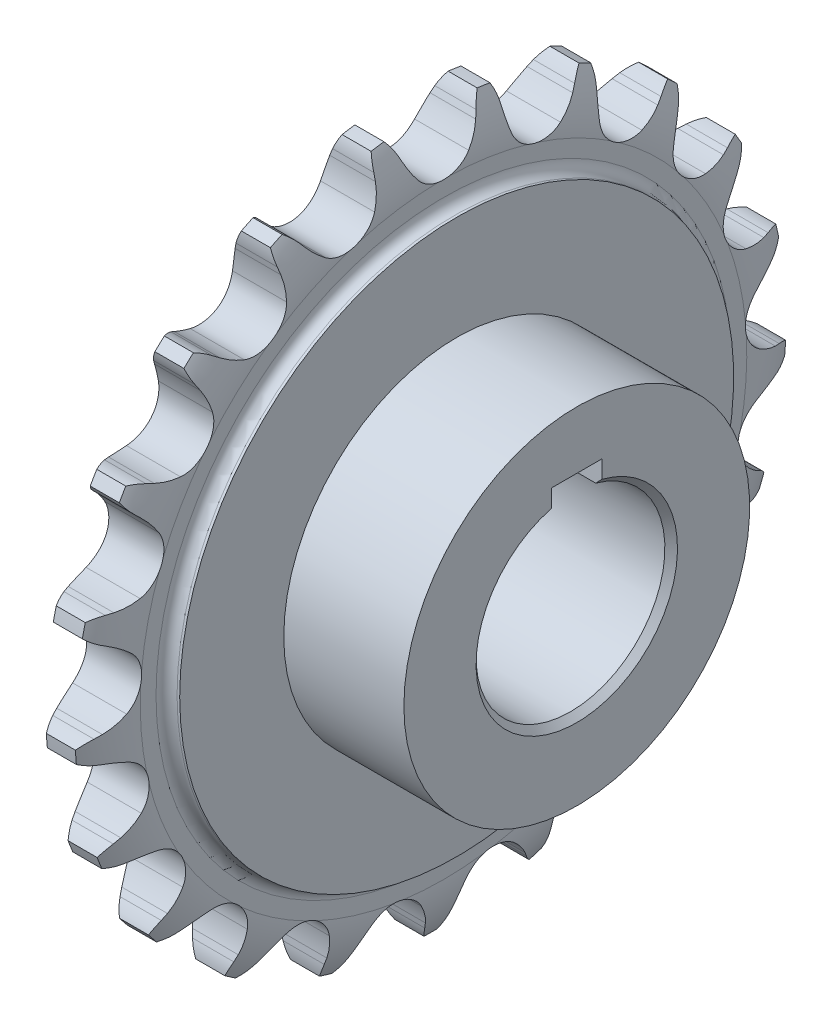
from build123d import *

# Parameters (mm, degrees)
CUT_EXTRUDE_1_DEPTH      = 6.459352492
PATTERN_CIRCULAR_1_COUNT = 21
SKETCH_3_W               = 19.081295016
SKETCH_3_H               = 12.4651341
SKETCH_4_W               = 8
SKETCH_4_H               = 3.843167657
CUT_EXTRUDE_2_DEPTH      = 87.013388292
CHAMFER_1_SIZE           = 1
CHAMFER_3_SIZE           = 1


with BuildPart() as part:
    # 草图1 → 旋转1 (revolve)
    with BuildSketch(Plane.XY, mode=Mode.PRIVATE) as revolve_1_sk:
        with BuildLine():
            Line((-6.459352492, 15), (-6.459352492, 44))
            Line((-6.459352492, 44), (-6.041681994, 44))
            ThreePointArc((-6.041681994, 44), (-4.860331427, 44.489331427), (-4.371, 45.670681994))
            Line((-4.371, 45.670681994), (-4.371, 48.176704985))
            ThreePointArc((-4.371, 48.176704985), (-3.911774122, 52.480340085), (-2.30725, 56.5))
            Line((-2.30725, 56.5), (2.30725, 56.5))
            ThreePointArc((2.30725, 56.5), (3.911774122, 52.480340085), (4.371, 48.176704985))
            Line((4.371, 48.176704985), (4.371, 45.670681994))
            ThreePointArc((4.371, 45.670681994), (4.860331427, 44.489331427), (6.041681994, 44))
            Line((6.041681994, 44), (6.459352492, 44))
            Line((6.459352492, 44), (6.459352492, 15))
            Line((6.459352492, 15), (-6.459352492, 15))
        make_face()
    revolve(revolve_1_sk.sketch.rotate(Axis((-7.9375, 0, 0), (1, 0, 0)), 90), axis=Axis((-7.9375, 0, 0), (1, 0, 0)))

    # 草图2 → 切除-拉伸1 (cut, symmetric)
    with BuildSketch(Plane(origin=(0, 0, 0), x_dir=(0, 0, -1), z_dir=(1, 0, 0))):
        with BuildLine():
            Line((5.852739584, 53.156379816), (6.249341137, 54.112736402))
            ThreePointArc((6.249341137, 54.112736402), (6.752605781, 55.10660921), (7.399855354, 56.013321101))
            ThreePointArc((7.399855354, 56.013321101), (0, 56.5), (-7.399855354, 56.013321101))
            ThreePointArc((-7.399855354, 56.013321101), (-6.752605781, 55.10660921), (-6.249341137, 54.112736402))
            Line((-6.249341137, 54.112736402), (-5.852739584, 53.156379816))
            ThreePointArc((-5.852739584, 53.156379816), (-5.064210074, 51.564909521), (-4.070411778, 50.09286284))
            ThreePointArc((-4.070411778, 50.09286284), (0, 48.101304985), (4.070411778, 50.09286284))
            ThreePointArc((4.070411778, 50.09286284), (5.064210074, 51.564909521), (5.852739584, 53.156379816))
        make_face()
    cut_extrude_1 = extrude(amount=CUT_EXTRUDE_1_DEPTH, both=True, mode=Mode.SUBTRACT)

    # 阵列(圆周)1: 切除-拉伸1 ×21 about axis
    pattern_circular_1_axis = Axis((0, 0, 0), (1, 0, 0))
    for i in range(1, PATTERN_CIRCULAR_1_COUNT):
        add(cut_extrude_1.rotate(pattern_circular_1_axis, i * 360 / PATTERN_CIRCULAR_1_COUNT), mode=Mode.SUBTRACT)

    # 草图3 → 旋转2 (revolve)
    with BuildSketch(Plane.XY, mode=Mode.PRIVATE) as revolve_2_sk:
        with Locations((16, 21.23256705)):
            Rectangle(SKETCH_3_W, SKETCH_3_H)
    revolve(revolve_2_sk.sketch.rotate(Axis((0, 0, 0), (1, 0, 0)), 90), axis=Axis((0, 0, 0), (1, 0, 0)))

    # 草图4 → 切除-拉伸2 (cut, through all)
    with BuildSketch(Plane.ZY.offset(6.459352492)):
        with Locations((0, 16.378416124)):
            Rectangle(SKETCH_4_W, SKETCH_4_H)
    extrude(amount=-CUT_EXTRUDE_2_DEPTH, mode=Mode.SUBTRACT)

    # 倒角1
    chamfer_1_edges = [part.edges().sort_by_distance(p)[0] for p in [
        (-6.459352492, -15, 0),
    ]]
    chamfer(chamfer_1_edges, length=CHAMFER_1_SIZE)

    # 倒角3
    chamfer_3_edges = [part.edges().sort_by_distance(p)[0] for p in [
        (25.540647508, -15, 0),
    ]]
    chamfer(chamfer_3_edges, length=CHAMFER_3_SIZE)


solid = part.part
